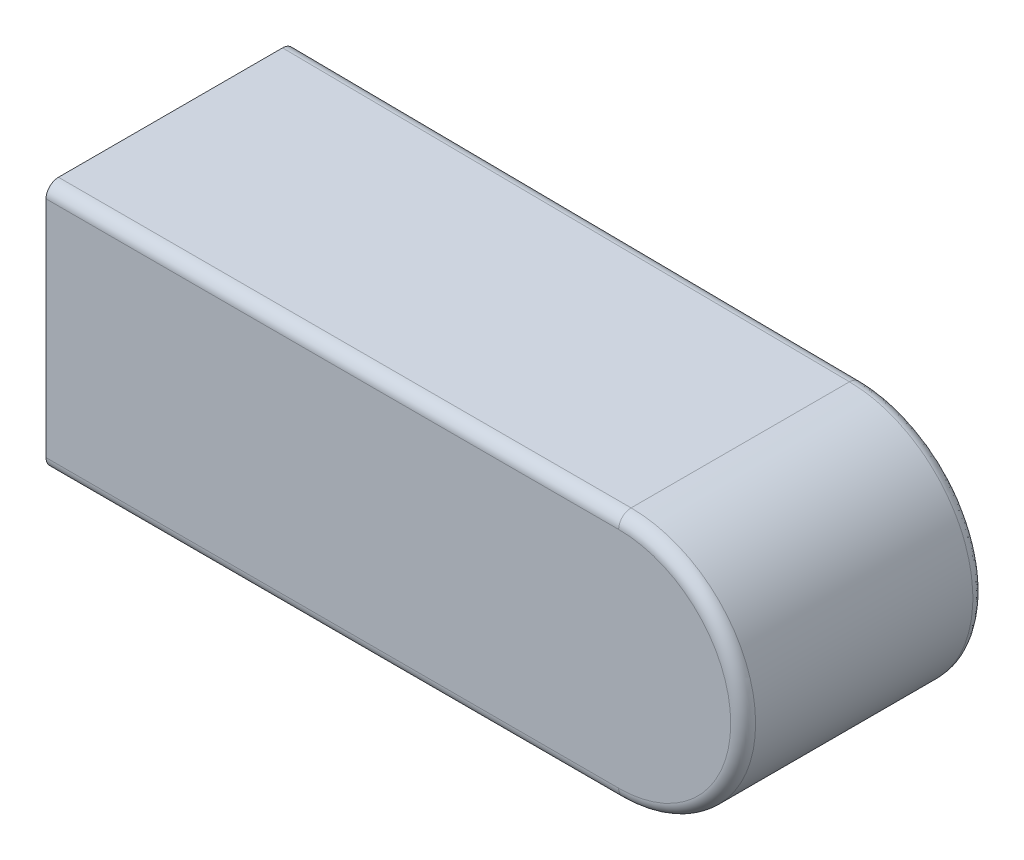
from build123d import *

# Parameters (mm, degrees)
EXTRUDE1_DEPTH          = 5
CUT_EXTRUDE1_DEPTH      = 9.958236434
CUT_EXTRUDE1_DEPTH_BACK = 9.958236434
FILLET2_R               = 0.25


with BuildPart() as part:
    # Sketch1 → Extrude1 (new body)
    with BuildSketch(Plane.XY):
        with BuildLine():
            Line((-7, 2.5), (4.5, 2.5))
            ThreePointArc((4.5, 2.5), (7, 0), (4.5, -2.5))
            Line((4.5, -2.5), (-7, -2.5))
            Line((-7, -2.5), (-7, 2.5))
        make_face()
    extrude(amount=EXTRUDE1_DEPTH)

    # Sketch2 → Cut-Extrude1 (cut, two sides: drawn at the far end of the back side and taken through both)
    with BuildSketch(Plane(origin=(0, 0, 0), x_dir=(1, 0, 0), z_dir=(0, 1, 0)).offset(-CUT_EXTRUDE1_DEPTH_BACK)):
        Polygon((-7, 0), (7, 0), (7, -0.14), align=None)
    extrude(amount=CUT_EXTRUDE1_DEPTH + CUT_EXTRUDE1_DEPTH_BACK, mode=Mode.SUBTRACT)

    # Fillet2
    fillet2_edges = [part.edges().sort_by_distance(p)[0] for p in [
        (7, 0, 5),
        (-1.25, 2.5, 5),
        (-1.25, -2.5, 0.0575),
        (6.267744857, -1.767789049, 0.132677449),
        (-1.25, 2.5, 0.0575),
        (-1.25, -2.5, 5),
    ]]
    fillet(fillet2_edges, radius=FILLET2_R)


solid = part.part
